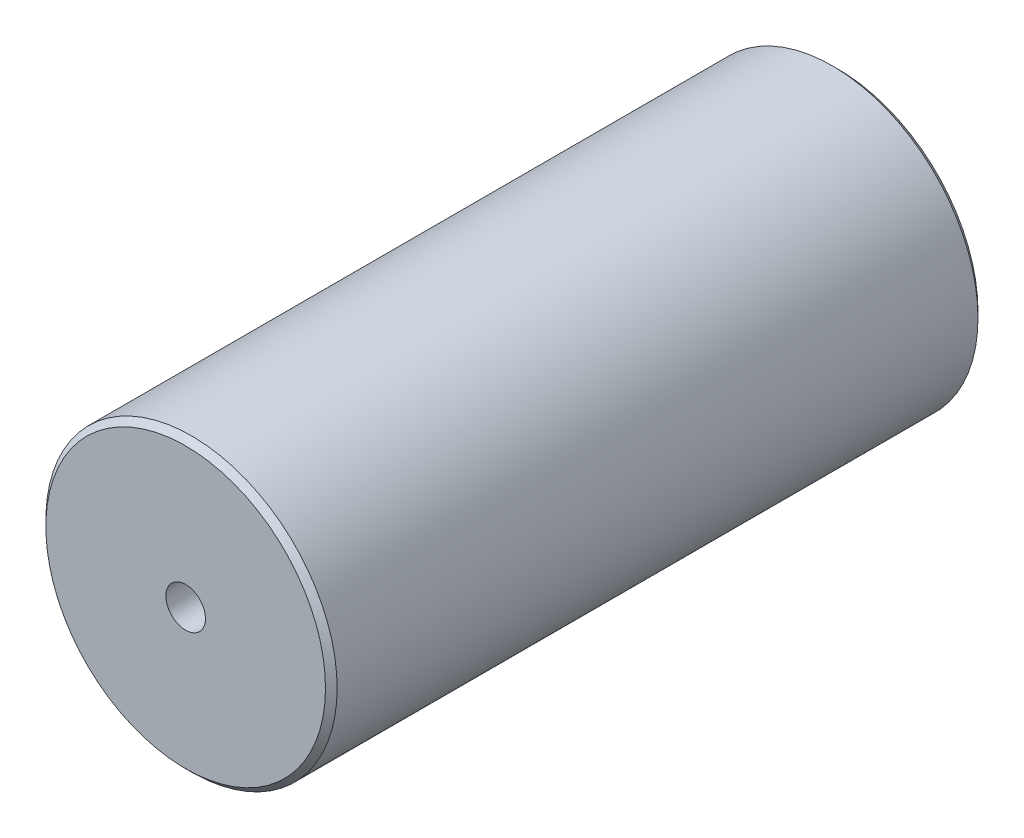
from build123d import *

# Parameters (mm, degrees)
SKETCH1_R             = 25
BOSS_EXTRUDE1_DEPTH   = 112
M8_TAPPED_HOLE1_D     = 6.8
M8_TAPPED_HOLE1_DEPTH = 22
M8_TAPPED_HOLE1_TIP   = 2.042926105
M8_TAPPED_HOLE2_D     = 6.8
M8_TAPPED_HOLE2_DEPTH = 23.75
M8_TAPPED_HOLE2_TIP   = 2.042926105
CHAMFER1_SIZE         = 1


with BuildPart() as part:
    # Sketch1 → Boss-Extrude1 (new body)
    with BuildSketch(Plane.XY):
        Circle(SKETCH1_R)
    extrude(amount=BOSS_EXTRUDE1_DEPTH)

    # M8 Tapped Hole1
    with Locations(Plane.XY.offset(112)):
        with Locations((0, 0)):
            Hole(M8_TAPPED_HOLE1_D / 2, depth=M8_TAPPED_HOLE1_DEPTH)
            with Locations((0, 0, -(M8_TAPPED_HOLE1_DEPTH + M8_TAPPED_HOLE1_TIP / 2))):  # 118° drill point
                Cone(0, M8_TAPPED_HOLE1_D / 2, M8_TAPPED_HOLE1_TIP, mode=Mode.SUBTRACT)

    # M8 Tapped Hole2
    with Locations(Plane(origin=(0, 0, 0), x_dir=(-1, 0, 0), z_dir=(0, 0, -1))):
        with Locations((0, 0)):
            Hole(M8_TAPPED_HOLE2_D / 2, depth=M8_TAPPED_HOLE2_DEPTH)
            with Locations((0, 0, -(M8_TAPPED_HOLE2_DEPTH + M8_TAPPED_HOLE2_TIP / 2))):  # 118° drill point
                Cone(0, M8_TAPPED_HOLE2_D / 2, M8_TAPPED_HOLE2_TIP, mode=Mode.SUBTRACT)

    # Chamfer1
    chamfer1_edges = [part.edges().sort_by_distance(p)[0] for p in [
        (-25, 0, 0),
        (-25, 0, 112),
    ]]
    chamfer(chamfer1_edges, length=CHAMFER1_SIZE)


solid = part.part
